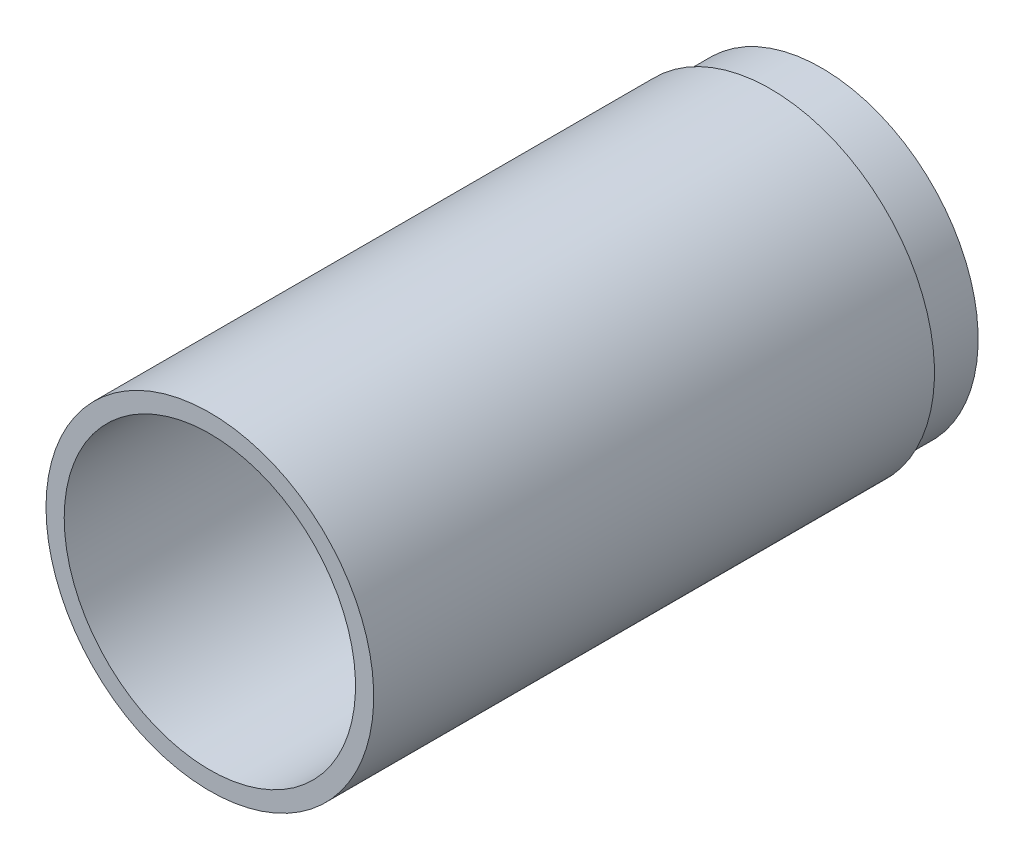
SolidWorks part; units mm, degrees
ref_plane "Front Plane" through (0, 0, 0) normal (0, 0, 1) x (1, 0, 0)
ref_plane "Top Plane" through (0, 0, 0) normal (0, 1, 0) x (1, 0, 0)
ref_plane "Right Plane" through (0, 0, 0) normal (1, 0, 0) x (0, 0, -1)
sketch "Sketch1" plane through (0, 0, 0) normal (0, 0, 1) x (1, 0, 0)
  circle A0 centre (0, 0) radius 22.5
  circle A1 centre (0, 0) radius 20
  dimension "D1" = 45
  dimension "D2" = 40
extrude "Boss-Extrude1" add sketch "Sketch1" along normal blind 84
sketch "Sketch2" plane through (0, 0, 0) normal (0, 0, -1) x (-1, 0, 0)
  circle A0 centre (0, 0) radius 21.5
  circle A1 centre (0, 0) radius 22.5
  dimension "D1" = 43
extrude "Cut-Extrude1" cut sketch "Sketch2" against normal blind 7
